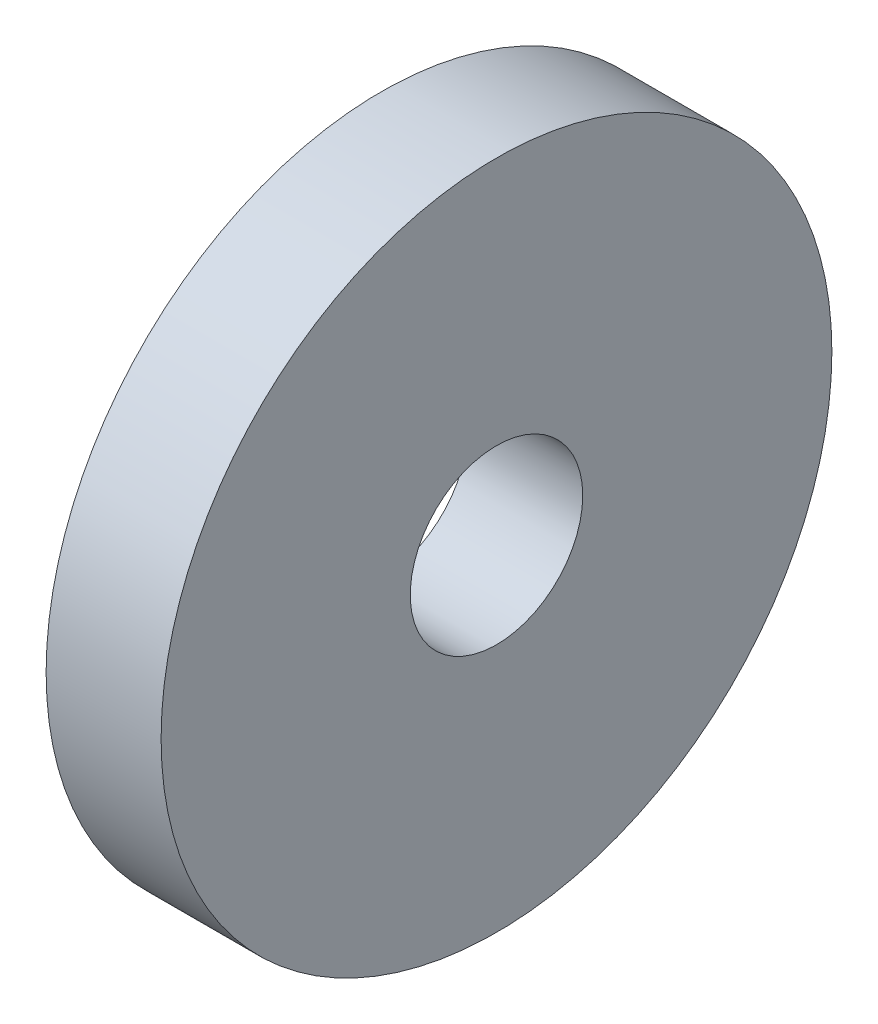
from build123d import *

# Parameters (mm, degrees)
SKETCH_1_R      = 17.5
SKETCH_1_R_2    = 4.5
EXTRUDE_1_DEPTH = 6


with BuildPart() as part:
    # 草图1 → 凸台-拉伸1 (new body)
    with BuildSketch(Plane(origin=(0, 0, 0), x_dir=(0, 0, -1), z_dir=(1, 0, 0))):
        Circle(SKETCH_1_R)
        Circle(SKETCH_1_R_2, mode=Mode.SUBTRACT)
    extrude(amount=EXTRUDE_1_DEPTH)


solid = part.part
